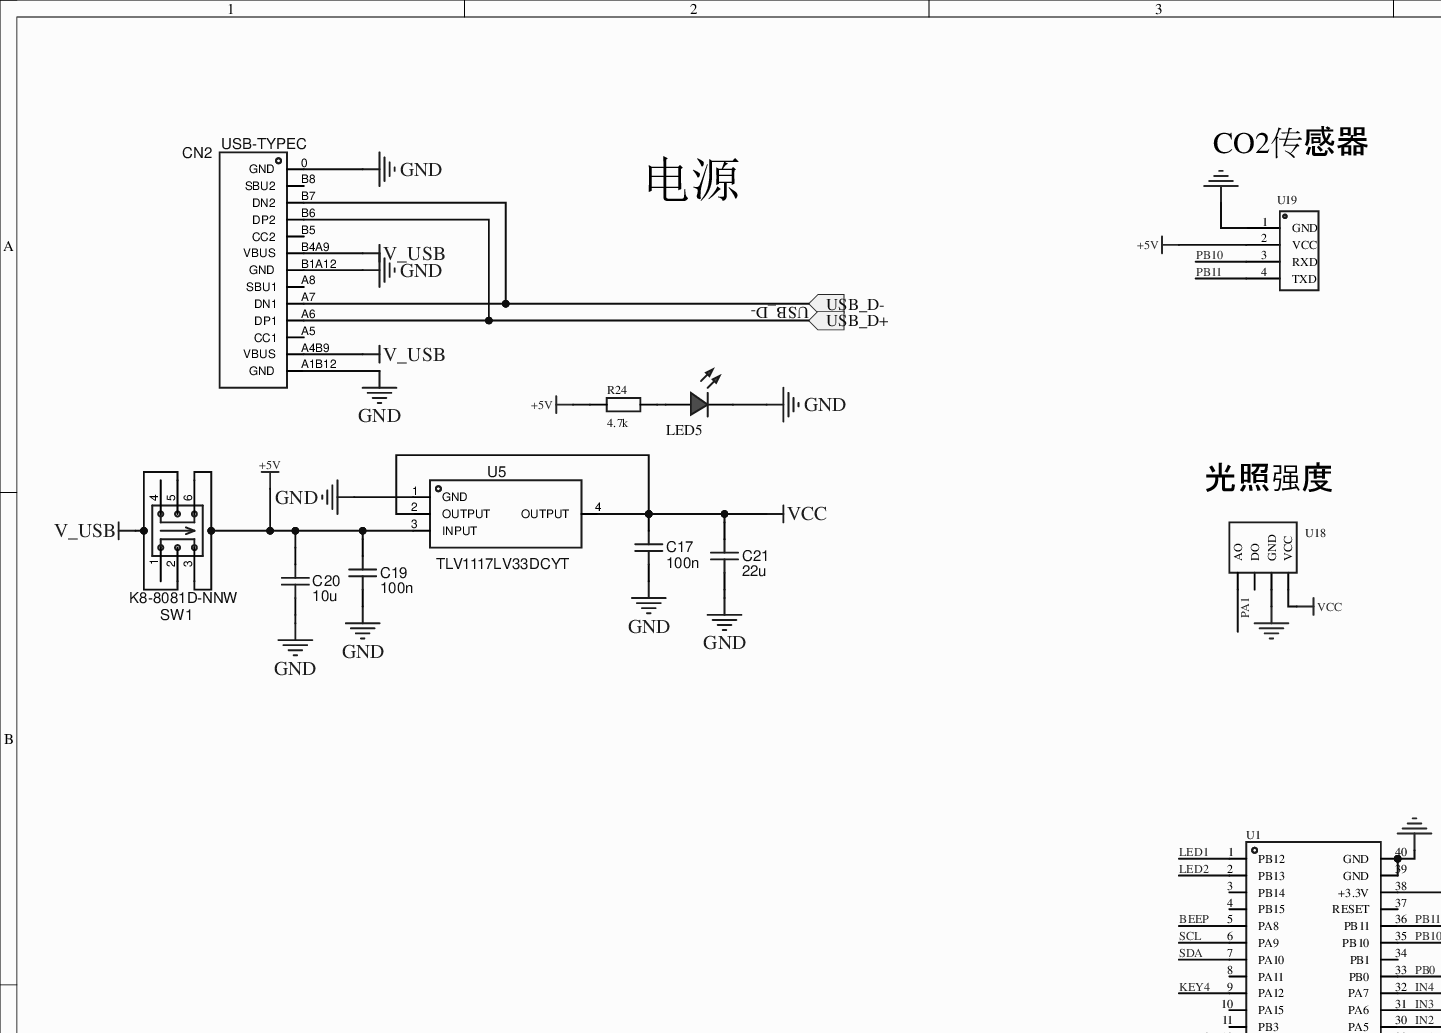
[diagram p0: MISC51844-3.schdoc, top left]
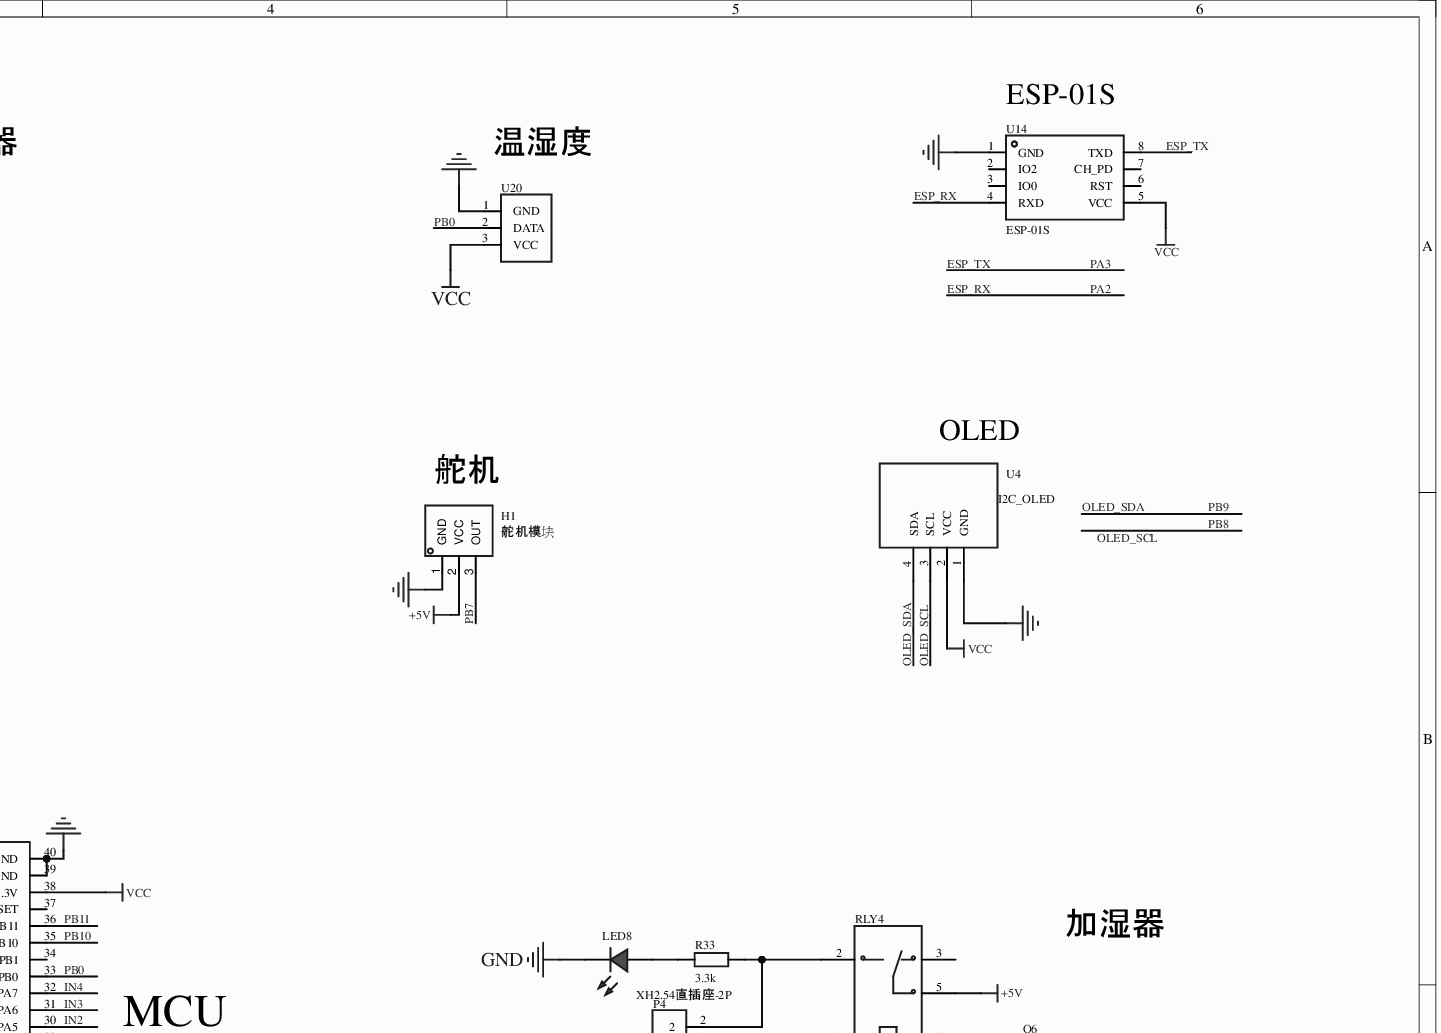
[diagram p1: MISC51844-3.schdoc, top right]
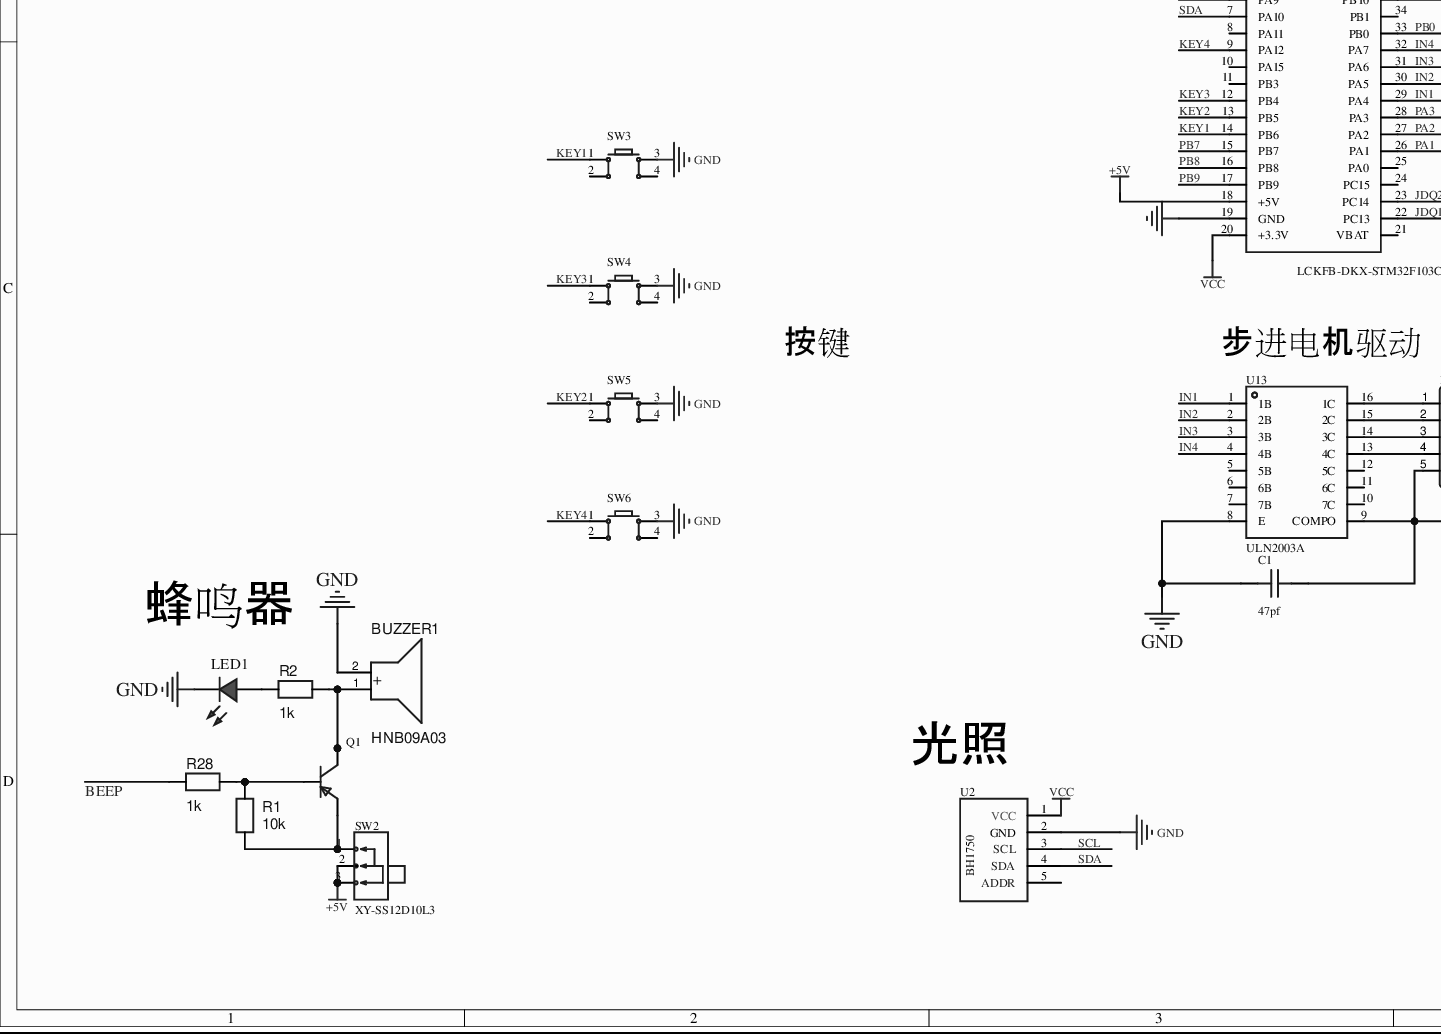
[diagram p2: MISC51844-3.schdoc, bottom left]
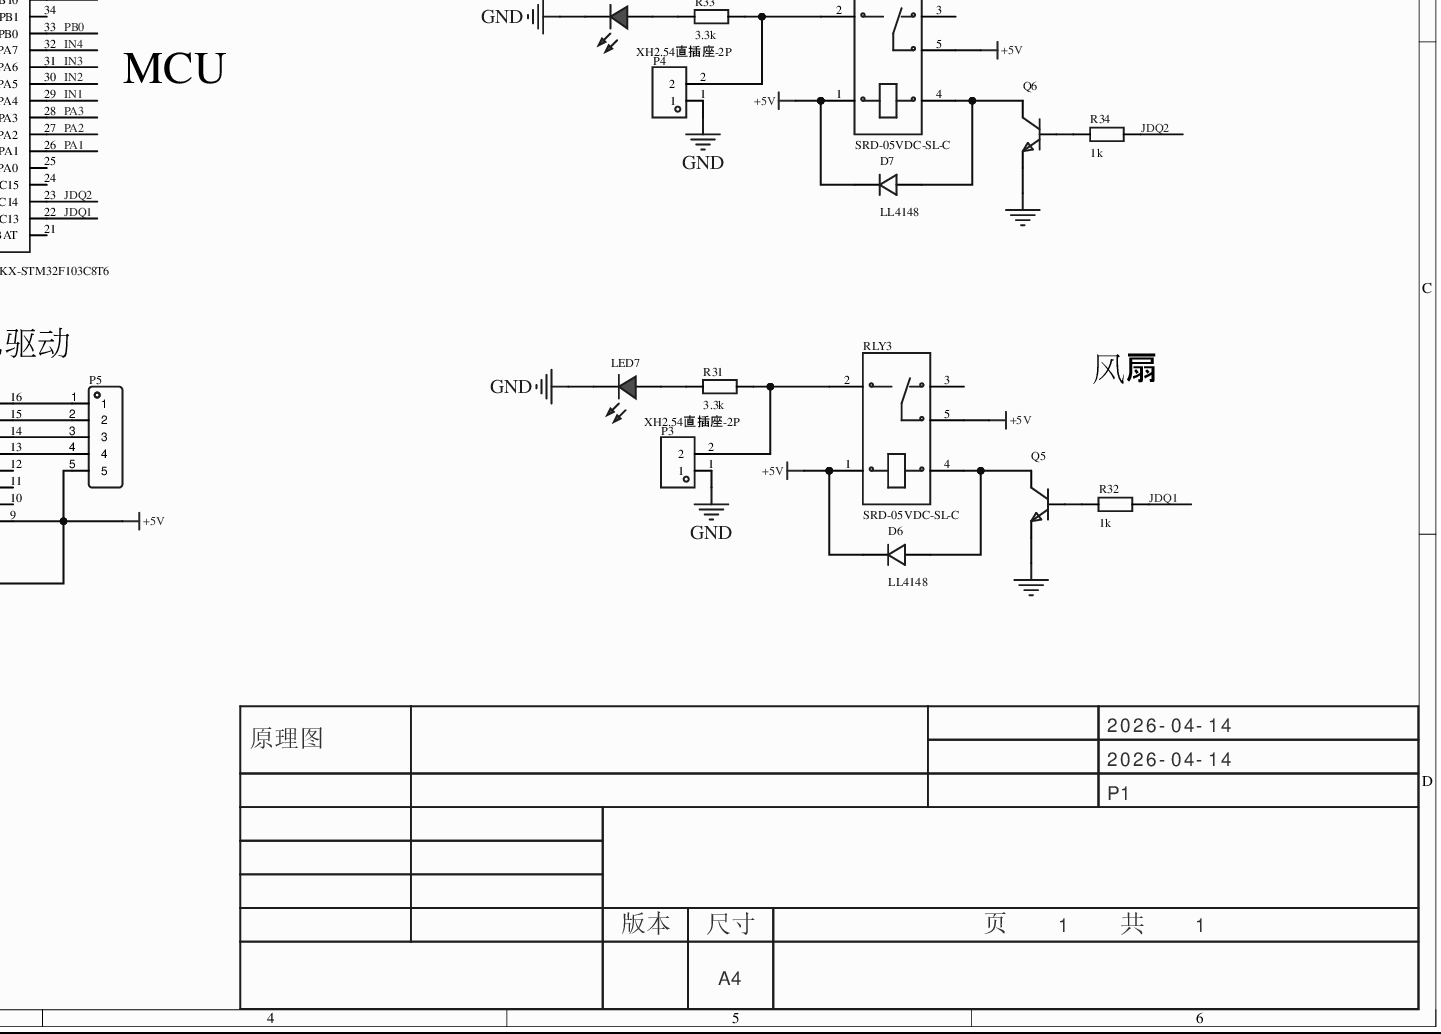
[diagram p3: MISC51844-3.schdoc, bottom right]
# Altium project MISC51844-2.PrjPcb
1 sheet, 45 parts. Net scope: flat (ports and power ports of the same name join across sheets).
Board file: MISC51844.pcbdoc

## Sheet MISC51844-3.schdoc
size 420 x 297 mm; Version: V1.0; @Project Name: MISC51844; @Update Date: 2026-04-14; @Create Date: 2026-04-14; @Board Name: MISC51844; @Create Time: 12:43:51; @Page Count: 1; @Page No: 1; @Schematic Name: MISC51844; @Update Time: 12:43:51; Size: A4

### Parts
BUZZER1  HNB09A03  [BUZ-TH_BD9.0-P5.00-D0.6-FD]
C1  47pf  [C0603]
C17  100n  [C0603]
C19  100n  [C0603]
C20  10u  [C0603]
C21  22u  [C0603]
CN2  USB-TYPEC  [USB-C-SMD_MC-307]
D6  LL4148  [LL-34_L3.5-W1.5-RD]
D7  LL4148  [LL-34_L3.5-W1.5-RD]
H1  舵机模块  [舵机模块]
LED1  (no value)  [LED_0603]
LED5  (no value)  [LED_0603]
LED7  (no value)  [LED_TH-3mm]
LED8  (no value)  [LED_TH-3mm]
P3  XH2.54直插座-2P  [CONN-TH_XH2.54-2P]
P4  XH2.54直插座-2P  [CONN-TH_XH2.54-2P]
P5  (no value)  [CONN-TH_XH2.54-5P]
Q1  (no value)  [S8550P_SOT]
Q5  (no value)  [S8050_SOT-23]
Q6  (no value)  [S8050_SOT-23]
R1  10k  [R0603]
R2  1k  [R0603]
R24  4.7k  [R0805]
R28  1k  [R0603]
R31  3.3k  [R0603]
R32  1k  [R0603]
R33  3.3k  [R0603]
R34  1k  [R0603]
RLY3  SRD-05VDC-SL-C  [RELAY-TH_SRD-XXVDC-XL-C]
RLY4  SRD-05VDC-SL-C  [RELAY-TH_SRD-XXVDC-XL-C]
SW1  K8-8081D-NNW  [SW-TH_6P-L8.0-W8.0-P2.50]
SW2  XY-SS12D10L3  [SW-TH_3P-L12.7-W6.7_XY-SS12D10LXX]
SW3  (no value)  [SW-TH_4P-L6.0-W6.0-P4.50-LS6.5]
SW4  (no value)  [SW-TH_4P-L6.0-W6.0-P4.50-LS6.5]
SW5  (no value)  [SW-TH_4P-L6.0-W6.0-P4.50-LS6.5]
SW6  (no value)  [SW-TH_4P-L6.0-W6.0-P4.50-LS6.5]
U1  LCKFB-DKX-STM32F103C8T6  [CONN-TH_L53.3-W22.9_STM32F103C8T6-CARD]
U2  (no value)  [BH1750光照传感器]
U4  (no value)  [OLED_I2C_0.96]
U5  TLV1117LV33DCYT  [SOT-223-4_L6.5-W3.5-P2.30-LS7.0-BR]
U13  ULN2003A  [SOP-16_L10.0-W3.9-P1.27-LS6.0-BL]
U14  ESP-01S  [WIFIM-TH_ESP-01S]
U18  光照强度模块  [光敏传感器]  (value not drawn)
U19  (no value)  [4P排母]
U20  (no value)  [dht11温湿度传感器]

### Ports
USB_D+ (in), USB_D- (in)

### Nets
+5V: C1.2 C19.2 C20.2 D6.1(K) D7.1(K) H1.2(VCC) P5.5 R24.1 RLY3.1 RLY3.5 RLY4.1 RLY4.5 SW1.3 SW1.6 SW2.2 SW2.3 U1.18(+5V) U5.3(INPUT) U13.9(COMPO) U19.2(VCC)
GND: BUZZER1.2(-) C1.1 C17.1 C19.1 C20.1 C21.1 CN2.0(GND) CN2.A1B12(GND) CN2.B1A12(GND) H1.1(GND) LED1.1(C) LED5.1(C) LED7.2(A) LED8.2(A) P3.1 P4.1 Q5.2 Q6.2 SW3.3 SW4.3 SW5.3 SW6.3 U1.19(GND) U1.39(GND) U1.40(GND) U2.2(GND) U4.1(GND) U5.1(GND) U13.8(E) U14.1(GND) U18.2(GND) U19.1(GND) U20.1(GND)
V_USB: CN2.A4B9(VBUS) CN2.B4A9(VBUS) SW1.2 SW1.5
VCC: C17.2 C21.2 U1.20(+3.3V) U1.38(+3.3V) U2.1(VCC) U4.2(VCC) U5.2(OUTPUT) U5.4(OUTPUT) U14.5(VCC) U18.1(VCC) U20.3(VCC)
BEEP: R28.1 U1.5(PA8)
ESP_RX: U1.27(PA2) U14.4(RXD)  [also labelled PA2]
ESP_TX: U1.28(PA3) U14.8(TXD)  [also labelled PA3]
IN1: U1.29(PA4) U13.1(1B)
IN2: U1.30(PA5) U13.2(2B)
IN3: U1.31(PA6) U13.3(3B)
IN4: U1.32(PA7) U13.4(4B)
JDQ1: R32.1 U1.22(PC13)
JDQ2: R34.1 U1.23(PC14)
KEY1: SW3.1 U1.14(PB6)
KEY2: SW5.1 U1.13(PB5)
KEY3: SW4.1 U1.12(PB4)
KEY4: SW6.1 U1.9(PA12)
LED1: U1.1(PB12)
LED2: U1.2(PB13)
OLED_SCL: U1.16(PB8) U4.3(SCL)  [also labelled PB8]
OLED_SDA: U1.17(PB9) U4.4(SDA)  [also labelled PB9]
PA1: U1.26(PA1) U18.4(AO)
PB0: U1.33(PB0) U20.2(DATA)
PB7: H1.3(OUT) U1.15(PB7)
PB10: U1.35(PB10) U19.3(RXD)
PB11: U1.36(PB11) U19.4(TXD)
SCL: U1.6(PA9) U2.3(SCL)
SDA: U1.7(PA10) U2.4(SDA)
USB_D-: CN2.A7(DN1) CN2.B7(DN2) ; port USB_D-
NetBUZZER1_1: BUZZER1.1(+) Q1.3(C) R2.2
NetCN2_A6: CN2.A6(DP1) CN2.B6(DP2) ; port USB_D+
NetD6_2: D6.2(A) Q5.3 RLY3.4
NetD7_2: D7.2(A) Q6.3 RLY4.4
NetLED1_2: LED1.2(A) R2.1
NetLED5_2: LED5.2(A) R24.2
NetLED7_1: LED7.1(C) R31.2
NetLED8_1: LED8.1(C) R33.2
NetP3_2: P3.2 R31.1 RLY3.2
NetP4_2: P4.2 R33.1 RLY4.2
NetP5_1: P5.1 U13.16(1C)
NetP5_2: P5.2 U13.15(2C)
NetP5_3: P5.3 U13.14(3C)
NetP5_4: P5.4 U13.13(4C)
NetQ1_1: Q1.1(B) R1.2 R28.2
NetQ1_2: Q1.2(E) R1.1 SW2.1
NetQ5_1: Q5.1 R32.2
NetQ6_1: Q6.1 R34.2

Not connected (* = marked no-connect by the designer): CN2 A5(CC1)* A8(SBU1)* B5(CC2)* B8(SBU2)*; RLY3 3*; RLY4 3*; SW1 1* 4*; SW3 2 4; SW4 2 4; SW5 2 4; SW6 2 4; U1 3(PB14) 4(PB15) 8(PA11) 10(PA15) 11(PB3) 21(VBAT) 24(PC15) 25(PA0) 34(PB1) 37(RESET); U2 5(ADDR); U13 5(5B) 6(6B) 7(7B) 10(7C) 11(6C) 12(5C); U14 2(IO2)* 3(IO0)* 6(RST)* 7(CH_PD)*; U18 3(DO)*

### Notes on the sheet
- CO2传感器
- (near U20) 温湿度
- (near U14) ESP-01S
- 电源
- 光照强度
- 舵机
- OLED
- 加湿器
- MCU
- 按键
- (near U13) 步进电机驱动
- 风扇
- 蜂鸣器
- 光照
- 2026-04-14
- 原理图
- P1
- 版本
- 尺寸
- A4
- 页    1    共    1

### Library data of the parts
BUZZER1 = HNB09A03: Manufacturer: 华能; Add into BOM: yes; Frequency: 3kHz; Symbol: HNB09A03; Device: HNB09A03; Convert to PCB: yes; Origin Footprint: BUZ-TH_BD9.0-P5.00-D0.6-FD; Supplier: LCSC; Supplier Part: C96102; Manufacturer Part: HNB09A03; JLCPCB Part Class: Extended Part; FootprintName: BUZ-TH_BD9.0-P5.00-D0.6-FD
C1 = CAP_0603: Symbol: CapAcitance; 3D Model: ac125912035d415993ca9572d50418b1; 3D Model Transform: 62.992,31.496,0,0,0,0,0,0,0; ConvertToPcb: yes; ModelName: C0603_L1.6-W0.8-H0.8; Device: CAP_0603; Value: 47pf; Supplier Footprint: 0603; AddInBom: yes; FootprintName: C0603
C17 C19-C21 = 100n: Add into BOM: yes; Symbol: 100n; Device: 100n; Convert to PCB: yes; Origin Footprint: C0603; FootprintName: C0603
CN2 = MC-307: Manufacturer: HANBO(汉博); Add into BOM: yes; Symbol: USB-TYPEC; Device: MC-307; Convert to PCB: yes; Origin Footprint: USB-C-SMD_MC-307; Supplier: LCSC; Supplier Part: C961709; Manufacturer Part: MC-307; JLCPCB Part Class: Extended Part; FootprintName: USB-C-SMD_MC-307
D6 D7 = LL4148_C9808: 二极管配置:-;功率:500mW;直流反向耐压(Vr):75V;平均整流电流(Io):200mA;正向压降(Vf):1V@10mA;反向电流(Ir):5uA@75V;反向恢复时间(trr):4ns;工作温度:+175℃@(Tj);; Manufacturer: ST(先科); 3D Model: 4a6f2309ca4c4217857da1816cccdf69; 3D Model Transform: 133.93674,59.031,0,0,0,0,0,0,0; Power Dissipation: 500mW; Reverse Voltage (Vr): 75V; Average Rectified Current (Io): 200mA; Reverse Recovery Time (trr): 4ns; AddInBom: yes; ModelName: LL-34_L3.5-W1.5; Symbol: LL4148; Device: LL4148_C9808; LCSC Part Name: 75V 200mA 4ns; Supplier Part: C9808; Manufacturer Part: LL4148; Supplier Footprint: LL-34; JLCPCB Part Class: 基础库; Datasheet: https://atta.szlcsc.com/upload/public/pdf/source/20121108/1457706554347.pdf; Supplier: LCSC; Diode Configuration: -; Forward Voltage (Vf@If): 1V@10mA; Reverse Leakage Current: 5uA@75V; Operating Temperature: +175℃@(Tj); ConvertToPcb: yes; FootprintName: LL-34_L3.5-W1.5-RD
H1 = 舵机模块: Manufacturer: Ckmtw(灿科盟); Manufacturer Part: B-2100S03P-A110; 3DModel: HDR-M-2.54_1x3; AddInBom: yes; Symbol: 舵机模块; Device: 舵机模块; link: https://item.szlcsc.com/50265.html; Supplier: LCSC; Supplier Part: C124376; ConvertToPcb: yes; FootprintName: 舵机模块
LED1 LED5 = LED_0603-R: Symbol: LED_R; Convert to PCB: yes; 3D Model: dd8257b0d61a4cd7b68939a056e08095; 3D Model Transform: 58.72,29.4,22.03,0,0,0,0,0,0; ModelName: LED-0603_R; Device: LED_0603-R; Add into BOM: yes; Supplier Footprint: 0603; FootprintName: LED_0603
LED7 LED8 = LED_TH-R_3mm: 3D Model: a497c992633541038a38947cdc58012f; 3D Model Transform: 141.274,153.327,0,0,0,0,-5.984,0,-137.795; ConvertToPcb: yes; ModelName: LED-TH-3mm_R; Symbol: LED_TH-R; Device: LED_TH-R_3mm; Supplier Footprint: 插件; AddInBom: yes; FootprintName: LED_TH-3mm
P3 P4 = XH2.54直插座-2P: 3D Model: dc9654a6caad4c20aab3bc231ea458cf; 3D Model Transform: 296.889,230.315,0,0,0,0,0,26.653,-137.795; AddInBom: yes; Symbol: XH2.54直插座-2P; Device: XH2.54直插座-2P; LCSC Part Name: XH2.54直插座-2P; Supplier Part: C9900016957; Manufacturer Part: XH2.54直插座-2P; Supplier Footprint: XH2.54-2; JLCPCB Part Class: 扩展库; Supplier: LCSC; ConvertToPcb: yes; FootprintName: CONN-TH_XH2.54-2P; ModelName: CONN-TH_XH2.54-2P
P5 = XH2.54-5P: Manufacturer: null; Manufacturer Part: XH-2.54-5P; AddInBom: yes; Symbol: XH2.54-5P; Device: XH2.54-5P; Supplier: LCSC; Supplier Part: C9900003918; ConvertToPcb: yes; FootprintName: CONN-TH_XH2.54-5P
Q1 = S8550_SOT_PNP: Symbol: PNP; ConvertToPcb: yes; ModelId: 9c0df02d6f3e44e889da37f3e5bf54960819f05c4eef4c71ace90d822a990e87; ModelName: SOT-23-3_L2.9-W1.4-P1.90-LS2.5-BR; ModelTransform: 98.43,114.17,37.91,0,0,0,0,0,0; Device: S8550_SOT_PNP; AddInBom: yes; Supplier Footprint: SOT-23; FootprintName: S8550P_SOT
Q5 Q6 = S8050_SOT_NPN: Symbol: NPN; 3D Model: c62791f0466c4ae2a892c056b845b0ca; 3D Model Transform: 98.6,114.12,41.29,180,0,0,0,0,-3; ConvertToPcb: yes; ModelName: SOT-23-3P_L2.9-W1.3-H1.0-LS2.4-P0.95; Device: S8050_SOT_NPN; Supplier Footprint: SOT-23; AddInBom: yes; FootprintName: S8050_SOT-23
R1 R2 R28 = 1k: Add into BOM: yes; Symbol: 1k; Device: 1k; Convert to PCB: yes; Origin Footprint: R0603; FootprintName: R0603
R24 = 0805W8F1002T5E_C17414: 电阻类型:厚膜电阻;阻值:10kΩ;精度:±1%;功率:125mW;; Manufacturer: UNI-ROYAL(厚声); 3D Model: 37a81e68749a4138bd2dfa6897b24b85; 3D Model Transform: 78.74,51.181,0,0,0,0,0,-0.0005,0; Tolerance: ±1%; Power(Watts): 125mW; Temperature Coefficient: ±100ppm/℃; Overload Voltage (Max): 150V; AddInBom: yes; ModelName: R0805_L2.0-W1.3-H0.6; Symbol: 0805W8F1002T5E; Device: 0805W8F1002T5E_C17414; Value: 4.7k; LCSC Part Name: 10kΩ ±1% 125mW; Manufacturer Part: 0805W8F1002T5E; Supplier Footprint: 0805; JLCPCB Part Class: 基础库; Datasheet: https://atta.szlcsc.com/upload/public/pdf/source/20200306/C422600_1E6D84923E4A46A82E41ADD87F860B5C.pdf; Supplier: LCSC; Type: 厚膜电阻; Operating Temperature Range: -55℃~+155℃; ConvertToPcb: yes; FootprintName: R0805
R31-R34 = Res_0603: Symbol: 电阻; 3D Model: fc143cca1e79419f9cd78b61e9279f08; 3D Model Transform: 31.8897,63.7794,0,90,0,0,0,0,0; ConvertToPcb: yes; Device: Res_0603; Supplier Footprint: 0603; AddInBom: yes; FootprintName: R0603; ModelName: R0603
  R31 R33: Value: 3.3k
  R32 R34: Value: 1k
RLY3 RLY4 = SRD-05VDC-SL-C: 线圈电压:5V;触点形式:一组转换:1C(单刀双掷-转换);触点容量(电阻负载):-;最大切换电压:250V@AC;最大切换电流:15A;; Manufacturer: 松乐; 3D Model: d0eda9b8bf8746d18ae810ab88dc78e7; 3D Model Transform: 755.904,622.4397,0,0,0,0,34.882,0,-118.11; Coil Voltage: 5V; Pin Number: 5; Coil Rated Power: 360mW; Maximum Switching Current: 15A; Coil Type: 无极性-单线圈; Coil Resistance: 70Ω; Contact Resistance: 100mΩ; Operate Time: 10ms; AddInBom: yes; ModelName: RELAY-TH_L19.2-W15.6-H15.8; Symbol: SRD-05VDC-SL-C; Device: SRD-05VDC-SL-C; LCSC Part Name: 蓝色; Supplier Part: C35449; Manufacturer Part: SRD-05VDC-SL-C; Supplier Footprint: 插件,15.6x19.2mm; JLCPCB Part Class: 扩展库; Datasheet: https://atta.szlcsc.com/upload/public/pdf/source/20200305/C490149_C96E4098A3B1FFB377D5AD2E40B7C2A8.pdf; Supplier: LCSC; Contact Form: 一组转换:1C(单刀双掷-转换); Contact Rating: -; Maximum Switching Voltage: 250V@AC; Release Time: 10ms; ConvertToPcb: yes; FootprintName: RELAY-TH_SRD-XXVDC-XL-C
SW1 = XKB8080-Z: Manufacturer: XKB Enterprise; Add into BOM: yes; Symbol: K8-8081D-NNW; Device: XKB8080-Z; Convert to PCB: yes; Origin Footprint: SW-TH_6P-L8.0-W8.0-P2.50; Supplier: LCSC; Supplier Part: C318860; Manufacturer Part: XKB8080-Z; FootprintName: SW-TH_6P-L8.0-W8.0-P2.50
SW2 = XY-SS12D10L3: 拨动开关,立式直脚两档,插件,单排正拨,柄长3mm; Manufacturer: XYECONN(辛译); AddInBom: yes; Symbol: XY-SS12D10L3; Device: XY-SS12D10L3; LCSC Part Name: 拨动开关,立式直脚两档,插件,单排正拨,柄长3mm; SupplierPart: C49652929; ManufacturerPart: XY-SS12D10L3; Supplier Footprint: 插件; JLCPCB Part Class: Extended Part; Datasheet: https://item.szlcsc.com/datasheet/XY-SS12D10L3/52215304.html; Supplier: LCSC; ConvertToPcb: yes; FootprintName: SW-TH_3P-L12.7-W6.7_XY-SS12D10LXX
SW3-SW6 = Key_TH_6x6x6: 触点电流:50mA;额定电压(DC):12V;绝缘电阻:100MΩ;电路结构:单刀单掷;安装方式:直插;按钮形状:圆形按钮;按钮/盖帽颜色:黑色;作用力:260gf@±30gf;工作温度:-25℃~+70℃;引脚样式:PC引脚;开关长度:6mm;开关宽度:6mm;开关高度:6mm;带支架:否;; Symbol: 轻触按键; AddInBom: yes; ModelId: 20eee248bc684ccd8cbdbb1d0d91ec6f0819f05c4eef4c71ace90d822a990e87; ModelName: SW-TH_4P-L6.0-W6.0-H5.0-LS6.5-P4.50; ModelTransform: 236.22,323.03,0,90,0,0,0,0,-137.795; Device: Key_TH_6x6x6; ConvertToPcb: yes; FootprintName: SW-TH_4P-L6.0-W6.0-P4.50-LS6.5; Supplier Footprint: 插件
U1 = LCKFB-DKX-STM32F103C8T6: Manufacturer: 立创开发板; AddInBom: yes; Symbol: LCKFB-DKX-STM32F103C8T6; Device: LCKFB-DKX-STM32F103C8T6; LCSC Part Name: 立创·地阔星-STM32F103C8T6开发板; Supplier Part: C22396880; Manufacturer Part: LCKFB-DKX-STM32F103C8T6; Supplier Footprint: -; JLCPCB Part Class: 扩展库; Datasheet: https://atta.szlcsc.com/upload/public/pdf/source/20240801/7EEF69F7480DF7C6DA98696664D658D4.pdf; Supplier: LCSC; ConvertToPcb: yes; FootprintName: CONN-TH_L53.3-W22.9_STM32F103C8T6-CARD
U2 = BH1750光照传感器: AddInBom: yes; Symbol: BH1750光照传感器; Device: BH1750光照传感器; ConvertToPcb: yes; FootprintName: BH1750光照传感器
U4 = I2C_OLED: 3D Model: 57daaad411c24bd7bd5d06edf5c4d16b0819f05c4eef4c71ace90d822a990e87; 3D Model Transform: 415.75,98.43,460.63,0,0,0,0,452.76,-118.11; ConvertToPcb: yes; ModelName: HDR-TH_4P-P2.54-F-LI-1X4P; Symbol: I2C_OLED; Device: I2C_OLED; AddInBom: yes; FootprintName: OLED_I2C_0.96
U5 = TLV1117LV33DCYT: Manufacturer: TI(德州仪器); Add into BOM: yes; Symbol: TLV1117LV33DCYT; Device: TLV1117LV33DCYT; Convert to PCB: yes; Origin Footprint: SOT-223-4_L6.5-W3.5-P2.30-LS7.0-BR; link: https://atta.szlcsc.comnull; Supplier: LCSC; Supplier Part: C2877977; Manufacturer Part: TLV1117LV33DCYT; JLCPCB Part Class: Extended Part; FootprintName: SOT-223-4_L6.5-W3.5-P2.30-LS7.0-BR
U13 = ULN2003A_C482013: 通道数:七路;集射击穿电压(Vceo):50V;; Manufacturer: UMW(友台半导体); 3D Model: 3361a6792abf4a8f8fbca4f1924a67ee; 3D Model Transform: 240.39054,393.7,0,90,0,0,0,0,0; number of channels: 七路; Maximum collector Emitter Voltage (Vceo): 50V; maximum input voltage: 30V; AddInBom: yes; ModelName: SOP-16_L9.9-W3.9-H1.5-LS6.0-P1.27; Symbol: ULN2003A_C482013; Device: ULN2003A_C482013; LCSC Part Name: ULN2003A; Supplier Part: C482013; Manufacturer Part: ULN2003A; Supplier Footprint: SOP-16; JLCPCB Part Class: Extended Part; Datasheet: https://atta.szlcsc.com/upload/public/pdf/source/20231109/03D8A8C909337F4ED8B7D0814C96A4D0.pdf; Supplier: LCSC; Operating Temperature: -40℃~+85℃; ConvertToPcb: yes; FootprintName: SOP-16_L10.0-W3.9-P1.27-LS6.0-BL
U14 = ESP-01S_C111009: 3D Model: eb7175da78ae48b3b1568cfe3027405f; 3D Model Transform: 582.676,976.37608,0,0,0,0,0,388.346,-118.11; AddInBom: yes; Symbol: ESP-01S; Device: ESP-01S_C111009; LCSC Part Name: ESP-01S; Supplier Part: C111009; Manufacturer Part: ESP-01S; Supplier Footprint: -; Supplier: LCSC; ConvertToPcb: yes; FootprintName: WIFIM-TH_ESP-01S; ModelName: WIFIM-TH_ESP-01S
U18 = 光照强度模块: ConvertToPcb: yes; Symbol: 光照强度模块; Device: 光照强度模块; Supplier Part: C115245; Supplier: LCSC; AddInBom: yes; FootprintName: 光敏传感器
U19 = 二氧化碳传感器: AddInBom: yes; Symbol: 二氧化碳传感器; Device: 二氧化碳传感器; ConvertToPcb: yes; FootprintName: 4P排母
U20 = DHT11: AddInBom: yes; Symbol: DHT11; Device: DHT11; ConvertToPcb: yes; FootprintName: dht11温湿度传感器